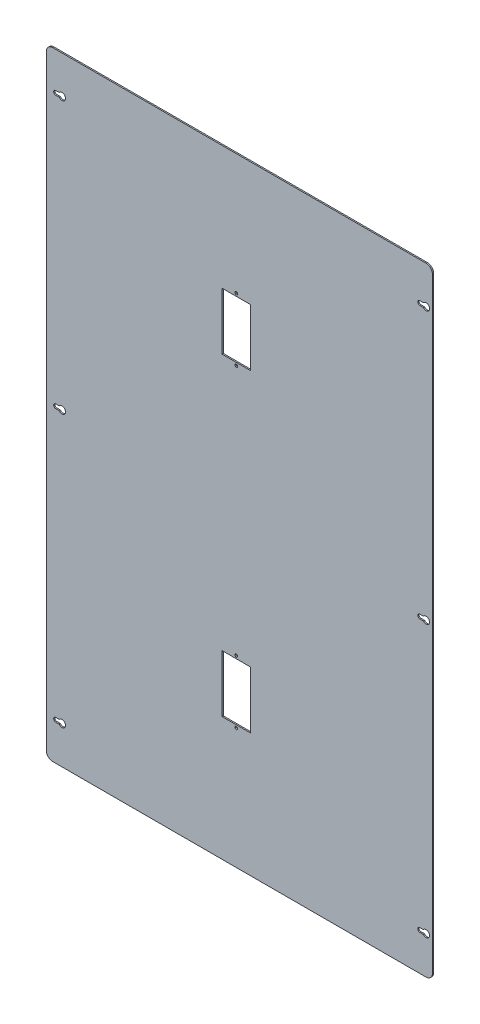
SolidWorks part; units mm, degrees
material "SPCC"
ref_plane "Front Plane" through (0, 0, 0) normal (0, 0, 1) x (1, 0, 0)
ref_plane "Top Plane" through (0, 0, 0) normal (0, 1, 0) x (1, 0, 0)
ref_plane "Right Plane" through (0, 0, 0) normal (1, 0, 0) x (0, 0, -1)
sketch "Sketch1" plane through (0, 0, 0) normal (0, 0, 1) x (1, 0, 0)
  line L1 (-307.5, 492.5) -> (307.5, 492.5)
  line L2 (-307.5, 492.5) -> (-307.5, -492.5)
  line L3 (-307.5, -492.5) -> (307.5, -492.5)
  line L4 (307.5, 492.5) -> (307.5, -492.5)
  line L5 (-307.5, 492.5) -> (307.5, -492.5) construction
  line L6 (-307.5, -492.5) -> (307.5, 492.5) construction
  point P0 (0, 0)
  dimension "D1" = 615
  dimension "D2" = 985
extrude "Boss-Extrude1" add sketch "Sketch1" along normal blind 2
sketch "Sketch7" plane through (0, 0, 0) normal (0, 0, -1) x (-1, 0, 0)
  line L1 (-17.5, 295.5) -> (27.5, 295.5)
  line L2 (-17.5, 295.5) -> (-17.5, 204.5)
  line L3 (-17.5, 204.5) -> (27.5, 204.5)
  line L4 (27.5, 295.5) -> (27.5, 204.5)
  line L5 (-17.5, 295.5) -> (27.5, 204.5) construction
  line L6 (-17.5, 204.5) -> (27.5, 295.5) construction
  line L7 (-17.5, -204.5) -> (27.5, -204.5)
  line L8 (-17.5, -204.5) -> (-17.5, -295.5)
  line L9 (-17.5, -295.5) -> (27.5, -295.5)
  line L10 (27.5, -204.5) -> (27.5, -295.5)
  line L11 (-17.5, -204.5) -> (27.5, -295.5) construction
  line L12 (-17.5, -295.5) -> (27.5, -204.5) construction
  point P0 (5, 250)
  point P5 (5, -250)
  dimension "D1" = 5
  dimension "D2" = 91
  dimension "D3" = 45
  dimension "D4" = 250
  dimension "D5" = 250
extrude "Cut-Extrude4" cut sketch "Sketch7" against normal through all
sketch "Sketch8" plane through (0, 0, 0) normal (0, 0, -1) x (-1, 0, 0)
  line L0 (5, -295.5) -> (5, -204.5) construction
  line L1 (-17.5, -295.5) -> (27.5, -295.5) construction
  line L2 (27.5, -204.5) -> (-17.5, -204.5) construction
  line L3 (-17.5, 204.5) -> (27.5, 204.5) construction
  circle A0 centre (5, 300) radius 2.25
  circle A1 centre (5, 200) radius 2.25
  circle A2 centre (5, -200) radius 2.25
  circle A3 centre (5, -300) radius 2.25
  dimension "D1" = 100
  dimension "D2" = 4.5
  dimension "D3" = 4.5
  dimension "D4" = 100
  dimension "D5" = 4.5
extrude "Cut-Extrude5" cut sketch "Sketch8" against normal through all
fillet "Fillet3" radius 10 4 edges at (307.5, -492.5, 1) (307.5, 492.5, 1) (-307.5, 492.5, 1) (-307.5, -492.5, 1)
sketch "Sketch10" plane through (0, 0, 0) normal (0, 0, -1) x (-1, 0, 0)
  line L0 (-297.5, 492.5) -> (297.5, 492.5) construction
  line L1 (307.5, 482.5) -> (307.5, -482.5) construction
  line L2 (292.5, 435.8) -> (286.9, 435.8)
  line L3 (292.5, 429.2) -> (286.9, 429.2)
  arc A0 (292.5, 429.2) -> (292.5, 435.8) centre (292.5, 432.5) ccw
  arc A1 (286.9, 435.8) -> (286.9, 429.2) centre (282.5, 432.5) ccw
  dimension "D4" = 11
  dimension "D5" = 6.6
  dimension "D1" = 60
  dimension "D2" = 15
  dimension "D3" = 10
extrude "Cut-Extrude6" cut sketch "Sketch10" against normal blind 10
pattern_linear "LPattern1" count 3 spacing 432.5 along (0, -1, 0) count 2 spacing 580 along (1, 0, 0) of "Cut-Extrude6"
sketch "Sketch11" plane through (0, 0, 2) normal (0, 0, 1) x (1, 0, 0)
  line L0 (-297.5, -492.5) -> (297.5, -492.5) construction
  line L1 (97.5, 517.5) -> (247.5, 517.5)
  line L2 (97.5, 517.5) -> (97.5, 267.5)
  line L3 (97.5, 267.5) -> (247.5, 267.5)
  line L4 (247.5, 517.5) -> (247.5, 267.5)
  line L5 (97.5, -182.5) -> (247.5, -182.5)
  line L6 (97.5, -182.5) -> (97.5, -412.5)
  line L7 (97.5, -412.5) -> (247.5, -412.5)
  line L8 (247.5, -182.5) -> (247.5, -412.5)
  line L9 (307.5, -482.5) -> (307.5, 482.5) construction
  dimension "D1" = 80
  dimension "D2" = 230
  dimension "D3" = 450
  dimension "D4" = 250
  dimension "D5" = 60
  dimension "D6" = 150
extrude "Cut-Extrude7" [suppressed] cut sketch "Sketch11" against normal through all
